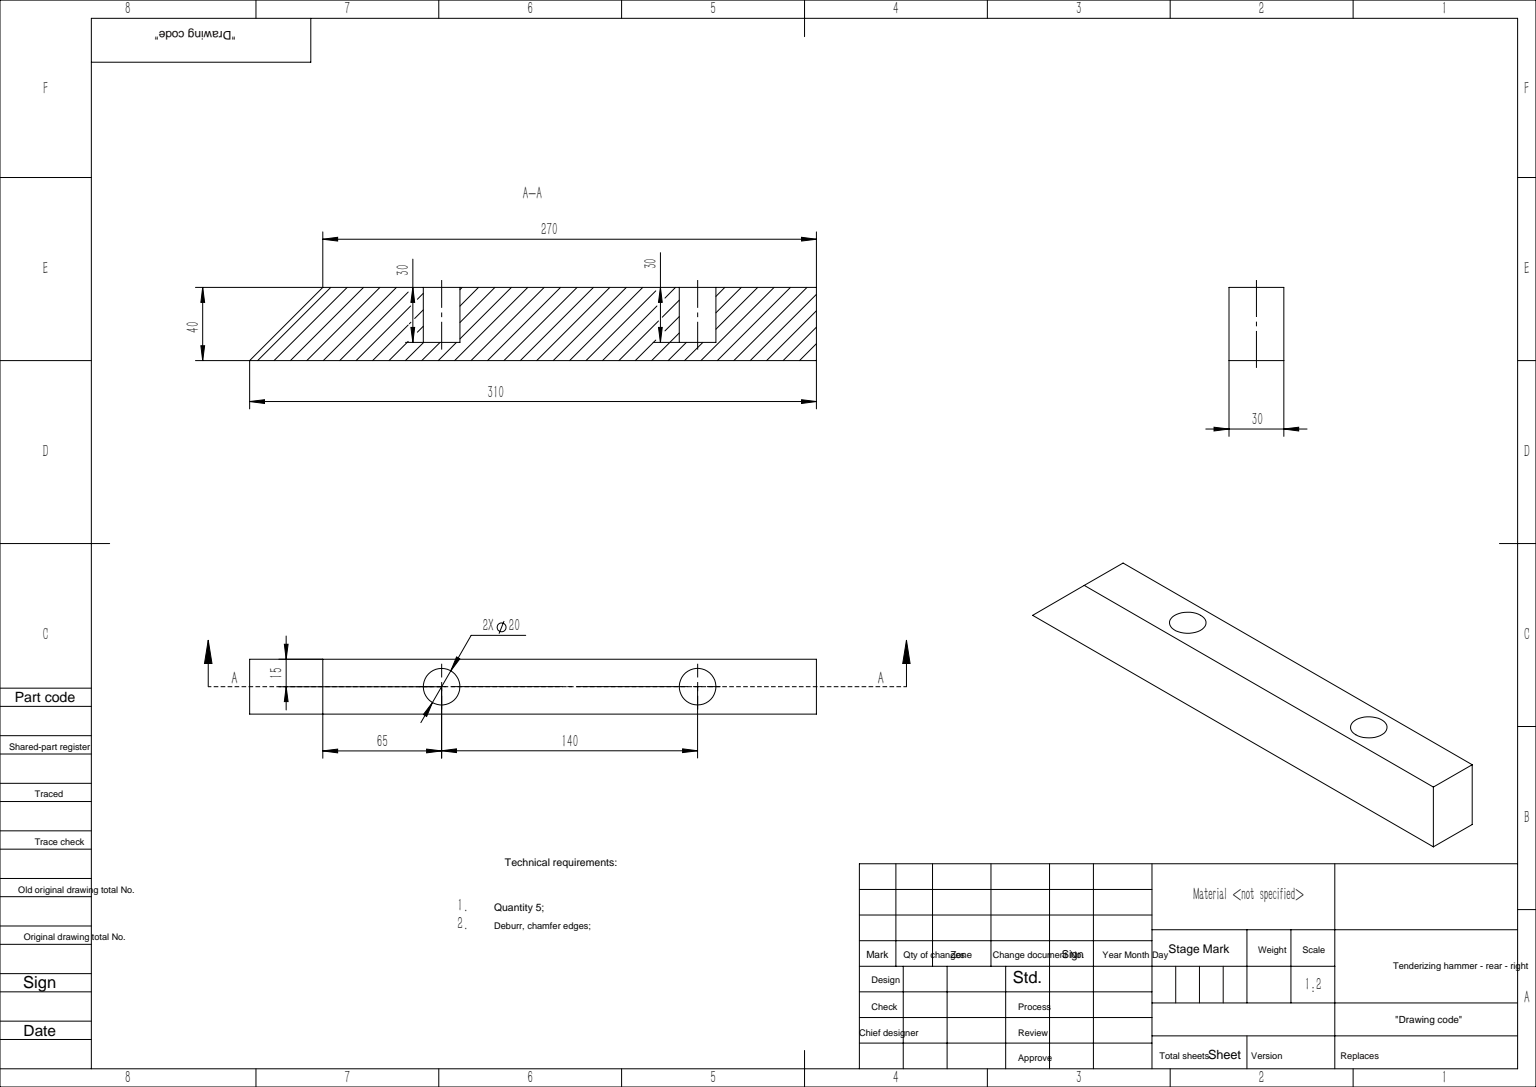
from build123d import *

# Parameters (mm, degrees)
SKETCH_1_W          = 270
SKETCH_1_H          = 30
EXTRUDE_1_DEPTH     = 40
SKETCH_2_R          = 10
CUT_EXTRUDE_2_DEPTH = 30
SKETCH_3_W          = 30
SKETCH_3_H          = 40
EXTRUDE_2_DEPTH     = 40
CUT_EXTRUDE_3_DEPTH = 183.002747232


with BuildPart() as part:
    # 草图1 → 凸台-拉伸1 (new body)
    with BuildSketch(Plane(origin=(0, 0, 0), x_dir=(1, 0, 0), z_dir=(0, 1, 0))):
        Rectangle(SKETCH_1_W, SKETCH_1_H)
    extrude(amount=EXTRUDE_1_DEPTH)

    # 草图2 → 切除-拉伸2 (cut)
    with BuildSketch(Plane(origin=(0, 40, 0), x_dir=(1, 0, 0), z_dir=(0, 1, 0))):
        with Locations(Location((70, 0, 0), (0, 0, 270))):
            Circle(SKETCH_2_R)
        with Locations(Location((-70, 0, 0), (0, 0, 90))):
            Circle(SKETCH_2_R)
    extrude(amount=-CUT_EXTRUDE_2_DEPTH, mode=Mode.SUBTRACT)

    # 草图3 → 凸台-拉伸2 (add)
    with BuildSketch(Plane.ZY.offset(135)):
        with Locations((0, 20)):
            Rectangle(SKETCH_3_W, SKETCH_3_H)
    extrude(amount=EXTRUDE_2_DEPTH)

    # 草图4 → 切除-拉伸3 (cut, through all)
    with BuildSketch(Plane.XY.offset(15)):
        Polygon((-175, 0), (-135, 40), (-175, 40), align=None)
    extrude(amount=-CUT_EXTRUDE_3_DEPTH, mode=Mode.SUBTRACT)


solid = part.part
